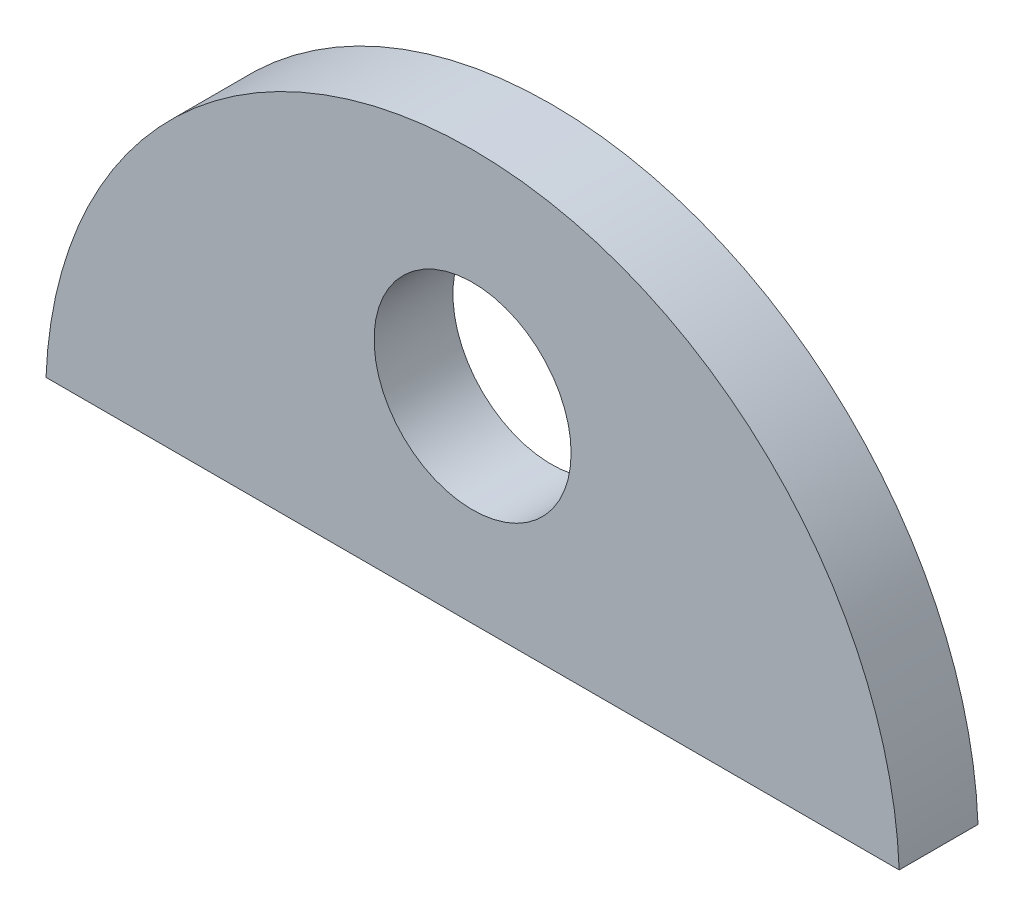
SolidWorks part; units mm, degrees
material "普通碳钢"
ref_plane "Front Plane" through (0, 0, 0) normal (0, 0, 1) x (1, 0, 0)
ref_plane "Top Plane" through (0, 0, 0) normal (0, 1, 0) x (1, 0, 0)
ref_plane "Right Plane" through (0, 0, 0) normal (1, 0, 0) x (0, 0, -1)
sketch "Sketch1" plane through (0, 0, 0) normal (0, 0, 1) x (1, 0, 0)
  line L0 (-129.9038, 5) -> (129.9038, 5)
  arc A0 (129.9038, 5) -> (-129.9038, 5) centre (0, 0) ccw
  circle A1 centre (0, 65) radius 30
  dimension "D1" = 260
  dimension "D3" = 60
  dimension "D2" = 5
  dimension "D4" = 60
extrude "Boss-Extrude1" add sketch "Sketch1" along normal mid plane 24
